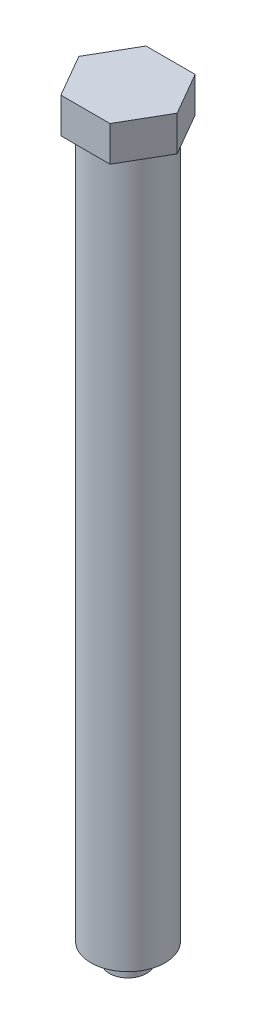
SolidWorks part; units mm, degrees
material "40Cr"
ref_plane "Front Plane" through (0, 0, 0) normal (0, 0, 1) x (1, 0, 0)
ref_plane "Top Plane" through (0, 0, 0) normal (0, 1, 0) x (1, 0, 0)
ref_plane "Right Plane" through (0, 0, 0) normal (1, 0, 0) x (0, 0, -1)
sketch "Sketch1" plane through (0, 0, 0) normal (0, 0, 1) x (1, 0, 0)
  line L0 (0, 0) -> (0, 152.5) construction
  line L1 (0, 0) -> (10, 0)
  line L2 (20, 10) -> (20, 391)
  line L3 (20, 391) -> (26.5, 391)
  line L4 (26.5, 391) -> (26.5, 410)
  line L5 (26.5, 410) -> (0, 410)
  line L6 (0, 410) -> (0, 0)
  line L7 (10, 0) -> (10, 10)
  line L8 (10, 10) -> (20, 10)
  dimension "D1" = 20
  dimension "D2" = 26.5
  dimension "D3" = 19
  dimension "D4" = 410
  dimension "D5" = 10
  dimension "D6" = 10
revolve "Revolve1" add sketch "Sketch1" angle 360 about L0
sketch "Sketch2" plane through (0, 410, 0) normal (0, 1, 0) x (1, 0, 0)
  line L1 (-26.5, 0) -> (-13.25, -22.9497)
  line L2 (-13.25, -22.9497) -> (13.25, -22.9497)
  line L3 (13.25, -22.9497) -> (26.5, 0)
  line L4 (26.5, 0) -> (13.25, 22.9497)
  line L5 (13.25, 22.9497) -> (-13.25, 22.9497)
  line L6 (-13.25, 22.9497) -> (-26.5, 0)
  circle A0 centre (0, 0) radius 22.9497 construction
  circle A1 centre (0, 0) radius 26.5 construction
extrude "Cut-Extrude1" cut sketch "Sketch2" against normal blind 32 flip side to cut
